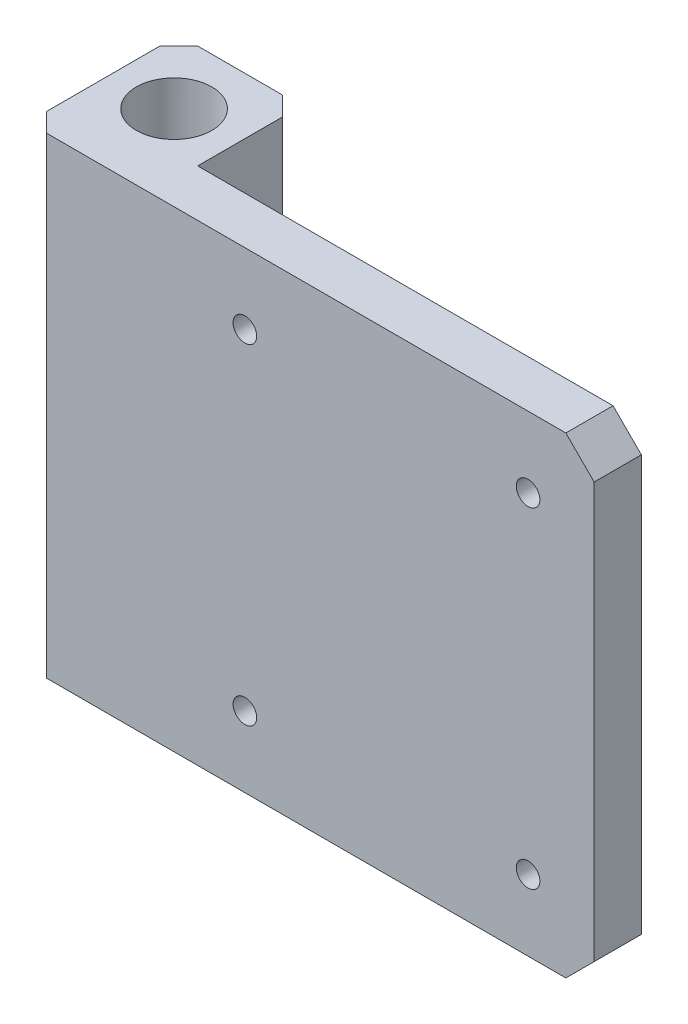
SolidWorks part; units mm, degrees
ref_plane "Front Plane" through (0, 0, 0) normal (0, 0, 1) x (1, 0, 0)
ref_plane "Top Plane" through (0, 0, 0) normal (0, 1, 0) x (1, 0, 0)
ref_plane "Right Plane" through (0, 0, 0) normal (1, 0, 0) x (0, 0, -1)
sketch "Sketch1" plane through (0, 0, 0) normal (0, 1, 0) x (1, 0, 0)
  line L1 (0, 0) -> (60, 0)
  line L2 (0, 0) -> (0, 16)
  line L3 (0, 16) -> (13, 16)
  line L4 (60, 0) -> (60, 5)
  line L7 (60, 5) -> (13, 5)
  line L8 (13, 16) -> (13, 5)
  dimension "D1" = 5
  dimension "D2" = 13
  dimension "D3" = 60
  dimension "D4" = 16
extrude "Boss-Extrude1" add sketch "Sketch1" along normal blind 50
sketch "Sketch2" plane through (0, 0, 0) normal (0, 0, 1) x (1, 0, 0)
  line L0 (0, 25) -> (50000, 25) construction
  line L1 (0, 50) -> (0, 0) construction
  line L2 (60, 50) -> (60, 0) construction
  circle A0 centre (53, 42.5) radius 0.75
  circle A1 centre (53, 7.5) radius 0.75
  point P4 (0, 25)
  dimension "D1" = 35
  dimension "D2" = 7
  dimension "D3" = 1.5
extrude "Cut-Extrude1" cut sketch "Sketch2" against normal blind 10
sketch "Sketch3" plane through (0, 50, 0) normal (0, 1, 0) x (1, 0, 0)
  line L0 (0, 0) -> (60, 0) construction
  line L1 (0, 16) -> (0, 0) construction
  circle A0 centre (6.5, 9) radius 4
  dimension "D1" = 8
  dimension "D2" = 9
  dimension "D3" = 6.5
extrude "Cut-Extrude2" cut sketch "Sketch3" against normal blind 60
chamfer "Chamfer1" distance 2 angle 45 3 edges at (0, 25, -16) (13, 25, -16) (0, 25, 0)
pattern_linear "LPattern1" count 2 spacing 30 along (-1, 0, 0) of "Cut-Extrude1"
chamfer "Chamfer2" distance 3 angle 45 2 edges at (60, 0, -2.5) (60, 50, -2.5)
hole_wizard "M3 Tapped Hole1" positions "3DSketch1" profile "Sketch4" tap size "M3" standard "Gb"
sketch3d "3DSketch1"
  line L0 (23, 42.5, -5) -> (23, 42.5, 0) construction
  line L1 (53, 42.5, -5) -> (53, 42.5, 0) construction
  line L2 (53, 7.5, -5) -> (53, 7.5, 0) construction
  line L3 (23, 7.5, -5) -> (23, 7.5, 0) construction
  point P0 (23, 42.5, 0)
  point P4 (53, 42.5, 0)
  point P8 (53, 7.5, 0)
  point P12 (23, 7.5, 0)
sketch "Sketch4" plane through (23, 42.5, 0) normal (1, 0, 0) x (0, -1, 0)
  line L0 (0, 0) -> (0, 8.2511)
  line L1 (0, 8.2511) -> (1.25, 7.5)
  line L2 (1.25, 7.5) -> (1.25, 0)
  line L5 (1.25, 0) -> (0, 0)
  line L10 (0, 8.2511) -> (-1.25, 7.5) construction
  line L11 (0, -6.35) -> (0, 107.95) construction
  dimension "螺纹孔钻头直径" = 2.5
  dimension "螺纹孔钻头深度" = 7.5
  dimension "导头角度" = 118
cosmetic thread "Hole Thread 1" parameters "D1"=5, "D2"=3
cosmetic thread "Hole Thread 2" parameters "D1"=5, "D2"=3
cosmetic thread "Hole Thread 3" parameters "D1"=5, "D2"=3
cosmetic thread "Hole Thread 4" parameters "D1"=5, "D2"=3
chamfer "Chamfer3" distance 0.8 angle 45 4 edges at (54.25, 7.5, -5) (24.25, 7.5, -5) (54.25, 42.5, -5) (24.25, 42.5, -5)
